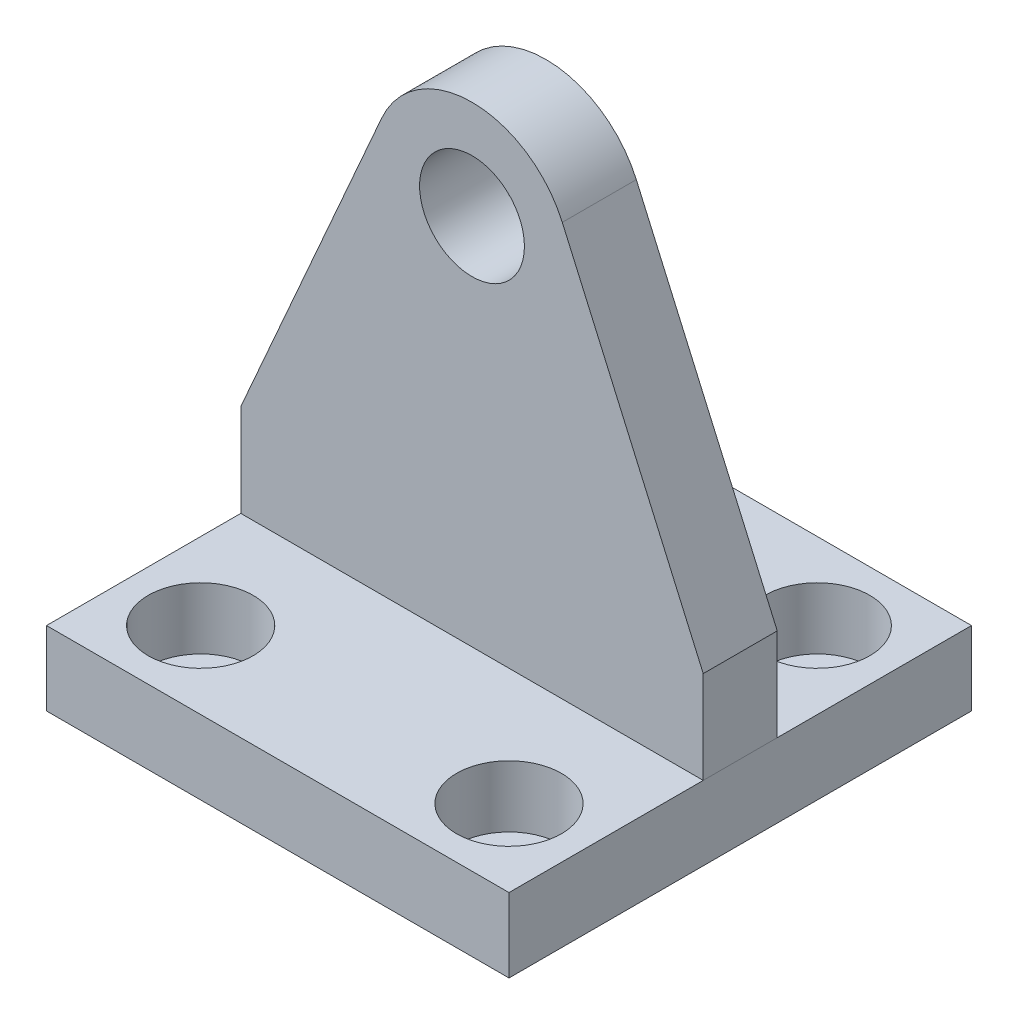
SolidWorks part; units mm, degrees
ref_plane "Front Plane" through (0, 0, 0) normal (0, 0, 1) x (1, 0, 0)
ref_plane "Top Plane" through (0, 0, 0) normal (0, 1, 0) x (1, 0, 0)
ref_plane "Right Plane" through (0, 0, 0) normal (1, 0, 0) x (0, 0, -1)
sketch "Sketch1" plane through (0, 0, 0) normal (0, 1, 0) x (1, 0, 0)
  line L1 (-37.5, 37.5) -> (37.5, 37.5)
  line L2 (-37.5, 37.5) -> (-37.5, -37.5)
  line L3 (-37.5, -37.5) -> (37.5, -37.5)
  line L4 (37.5, 37.5) -> (37.5, -37.5)
  line L5 (-37.5, 37.5) -> (37.5, -37.5) construction
  line L6 (-37.5, -37.5) -> (37.5, 37.5) construction
  point P0 (0, 0)
  dimension "D1" = 75
  dimension "D2" = 75
extrude "Boss-Extrude1" add sketch "Sketch1" along normal blind 12
sketch "Sketch2" plane through (0, 12, 0) normal (0, 1, 0) x (1, 0, 0)
  line L0 (37.5, -37.5) -> (37.5, 37.5) construction
  line L1 (-37.5, 6) -> (37.5, 6)
  line L2 (-37.5, 6) -> (-37.5, -6)
  line L3 (-37.5, -6) -> (37.5, -6)
  line L4 (37.5, 6) -> (37.5, -6)
  line L5 (-37.5, 6) -> (37.5, -6) construction
  line L6 (-37.5, -6) -> (37.5, 6) construction
  point P0 (0, 0)
  dimension "D1" = 12
extrude "Boss-Extrude2" add sketch "Sketch2" along normal blind 76.5 separate body
sketch "Sketch3" plane through (0, 0, 6) normal (0, 0, 1) x (1, 0, 0)
  line L0 (0, 0) -> (0, 88.5) construction
  line L1 (-37.5, 88.5) -> (37.5, 88.5) construction
  line L2 (-37.5, 12) -> (37.5, 12) construction
  circle A0 centre (0, 72.5) radius 8.5
  dimension "D1" = 60.5
  dimension "D2" = 17
extrude "Cut-Extrude1" cut sketch "Sketch3" against normal through all
sketch "Sketch4" plane through (0, 0, 6) normal (0, 0, 1) x (1, 0, 0)
  line L0 (-37.5, 27) -> (-14.6451, 78.9437)
  line L1 (-37.5, 88.5) -> (-37.5, 12) construction
  line L2 (-37.5, 88.5) -> (37.5, 88.5) construction
  line L3 (-37.5, 27) -> (-37.5, 88.5)
  line L4 (-37.5, 88.5) -> (-37.5, 96.342)
  line L5 (0, 0) -> (0, 88.5) construction
  line L6 (37.5, 27) -> (37.5, 88.5)
  line L7 (37.5, 27) -> (14.6451, 78.9437)
  line L8 (-37.5, 96.342) -> (37.5, 96.342)
  line L9 (37.5, 96.342) -> (37.5, 88.5)
  arc A0 (14.6451, 78.9437) -> (-14.6451, 78.9437) centre (0, 72.5) ccw
  dimension "D1" = 15
extrude "Cut-Extrude2" cut sketch "Sketch4" against normal through all
hole_wizard "CBORE for M10 Hex Head Bolt2" positions "Sketch5" profile "Sketch6" counterbore size "M10" standard "GB"
sketch "Sketch5" plane through (0, 12, 0) normal (0, 1, 0) x (1, 0, 0)
  line L0 (0, 37.5) -> (0, -37.5) construction
  line L1 (37.5, 37.5) -> (-37.5, 37.5) construction
  line L2 (-37.5, -37.5) -> (37.5, -37.5) construction
  line L4 (-37.5, 0) -> (37.5, 0) construction
  line L5 (-37.5, 37.5) -> (-37.5, -37.5) construction
  line L6 (37.5, 6) -> (37.5, -6) construction
  line L9 (-25, 25) -> (25, 25) construction
  line L10 (-25, 25) -> (-25, -25) construction
  line L11 (-25, -25) -> (25, -25) construction
  line L12 (25, 25) -> (25, -25) construction
  line L13 (-25, 25) -> (25, -25) construction
  line L14 (-25, -25) -> (25, 25) construction
  point P16 (25, -25)
  point P191 (-25, 25)
  point P192 (-25, -25)
  point P193 (25, 25)
  point P196 (0, 0)
  dimension "D1" = 50
  dimension "D2" = 50
sketch "Sketch6" plane through (25, 12, 25) normal (1, 0, 0) x (0, 0, 1)
  line L0 (0, 0) -> (0, 46.8047)
  line L1 (0, 46.8047) -> (5.5, 43.5)
  line L2 (5.5, 43.5) -> (5.5, 10)
  line L3 (5.5, 10) -> (8.5, 10)
  line L4 (8.5, 10) -> (8.5, 0)
  line L5 (8.5, 0) -> (0, 0)
  line L10 (0, 46.8047) -> (-5.5, 43.5) construction
  line L11 (0, -6.35) -> (0, 107.95) construction
  dimension "孔直径" = 11
  dimension "孔深度" = 43.5
  dimension "柱形沉头孔直径" = 17
  dimension "柱形沉头孔深度" = 10
  dimension "导头角度" = 118
